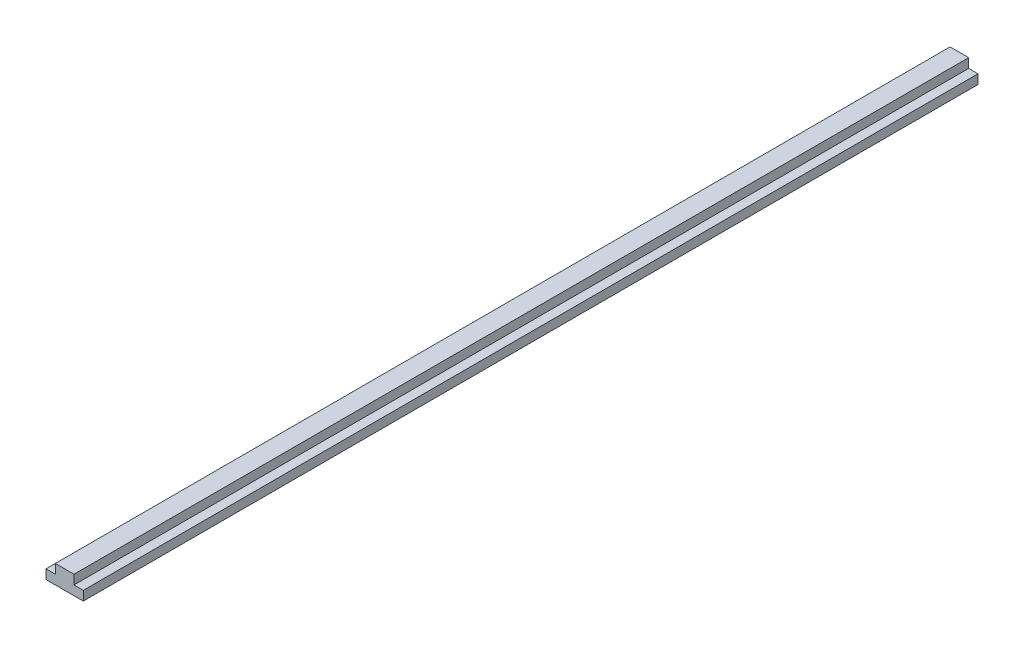
SolidWorks part; units mm, degrees
ref_plane "Front Plane" through (0, 0, 0) normal (0, 0, 1) x (1, 0, 0)
ref_plane "Top Plane" through (0, 0, 0) normal (0, 1, 0) x (1, 0, 0)
ref_plane "Right Plane" through (0, 0, 0) normal (1, 0, 0) x (0, 0, -1)
other "Configuration Table"
sketch "Sketch1" plane through (0, 0, 0) normal (0, 0, 1) x (1, 0, 0)
  line L0 (5, 5) -> (5, 10)
  line L1 (0, 0) -> (20, 0)
  line L2 (0, 0) -> (0, 5)
  line L3 (0, 5) -> (5, 5)
  line L4 (20, 0) -> (20, 5)
  line L5 (5, 10) -> (15, 10)
  line L6 (15, 10) -> (15, 5)
  line L7 (15, 5) -> (20, 5)
  dimension "D1" = 20
  dimension "D2" = 5
  dimension "D3" = 10
  dimension "D4" = 5
  dimension "D5" = 5
extrude "Boss-Extrude1" add sketch "Sketch1" along normal blind 480
